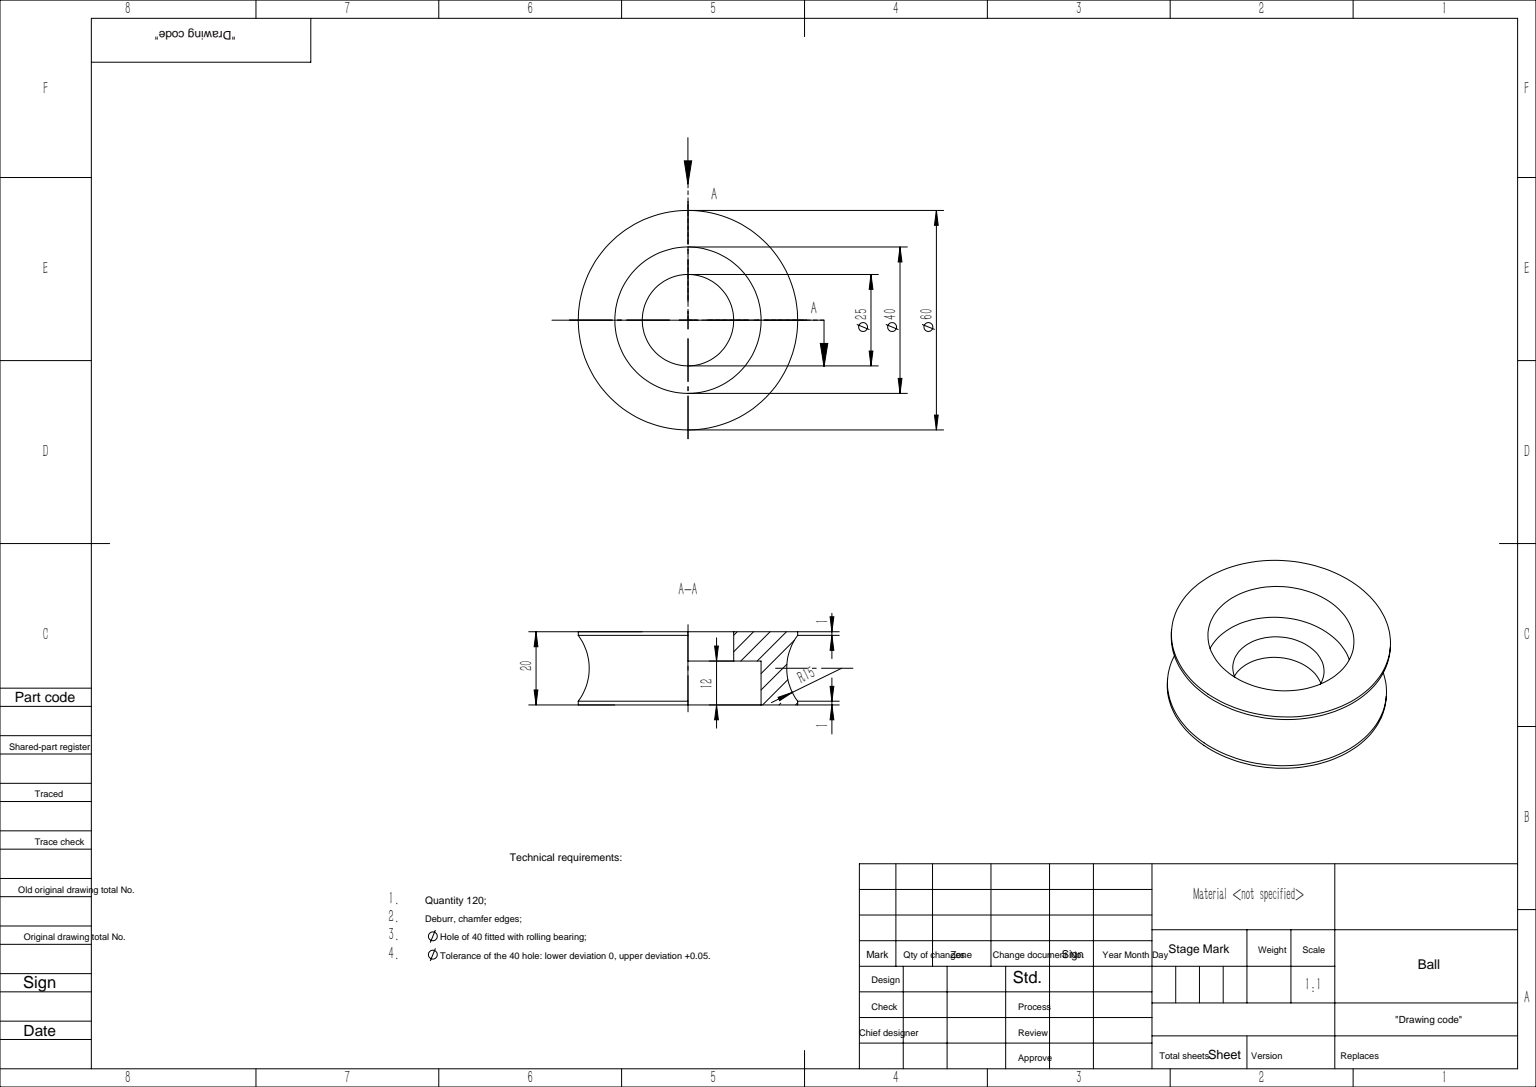
from build123d import *

# Parameters (mm, degrees)
SKETCH_1_R               = 30
EXTRUDE_1_DEPTH          = 20
SKETCH_2_R               = 20
CUT_EXTRUDE_1_DEPTH      = 12
CUT_EXTRUDE_2_DEPTH      = 45.09081537
CUT_EXTRUDE_2_DEPTH_BACK = 45.09081537
SKETCH_4_R               = 12.5
SKETCH_5_R               = 15


with BuildPart() as part:
    # 草图1 → 凸台-拉伸1 (new body)
    with BuildSketch(Plane(origin=(0, 0, 0), x_dir=(1, 0, 0), z_dir=(0, 1, 0))):
        with Locations(Location((0, 0, 0), (0, 0, 270))):
            Circle(SKETCH_1_R)
    extrude(amount=EXTRUDE_1_DEPTH)

    # 草图2 → 切除-拉伸1 (cut)
    with BuildSketch(Plane(origin=(0, 20, 0), x_dir=(1, 0, 0), z_dir=(0, 1, 0))):
        with Locations(Location((0, 0, 0), (0, 0, 270))):
            Circle(SKETCH_2_R)
    extrude(amount=-CUT_EXTRUDE_1_DEPTH, mode=Mode.SUBTRACT)

    # 草图4 → 切除-拉伸2 (cut, two sides: drawn at the far end of the back side and taken through both)
    with BuildSketch(Plane(origin=(0, 8, 0), x_dir=(1, 0, 0), z_dir=(0, 1, 0)).offset(-CUT_EXTRUDE_2_DEPTH_BACK)):
        with Locations(Location((0, 0, 0), (0, 0, 270))):
            Circle(SKETCH_4_R)
    extrude(amount=CUT_EXTRUDE_2_DEPTH + CUT_EXTRUDE_2_DEPTH_BACK, mode=Mode.SUBTRACT)

    # 草图5 → 切除-旋转1 (revolve, cut)
    with BuildSketch(Plane.XY, mode=Mode.PRIVATE) as cut_revolve_1_sk:
        with Locations((42, 10)):
            Circle(SKETCH_5_R)
    revolve(cut_revolve_1_sk.sketch.rotate(Axis((0, 0, 0), (0, 1, 0)), 90), axis=Axis((0, 0, 0), (0, 1, 0)), mode=Mode.SUBTRACT)


solid = part.part
